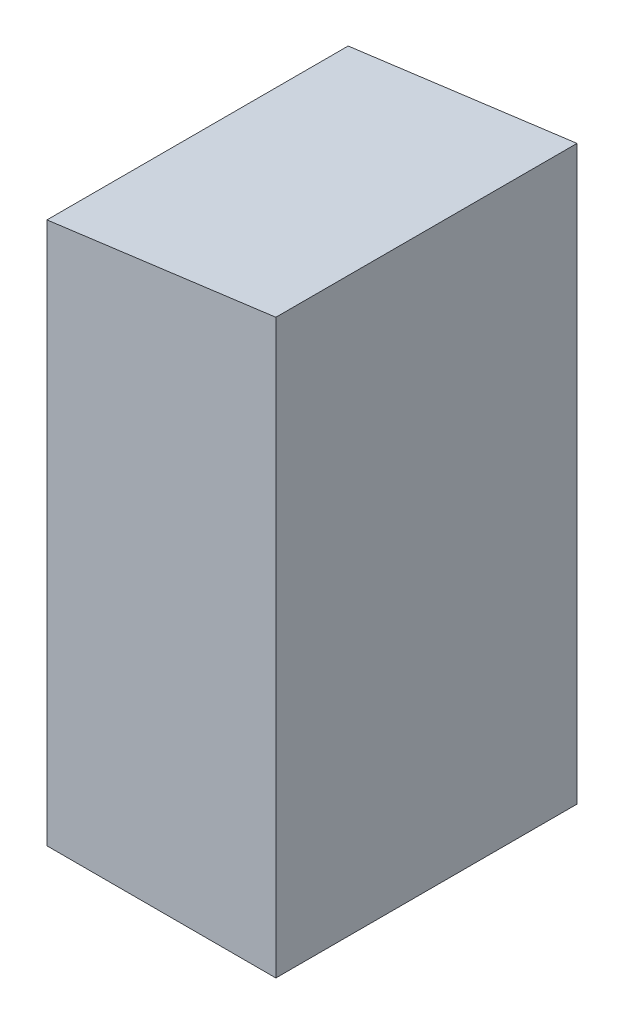
from build123d import *

# Parameters (mm, degrees)
BOSS_EXTRUDE1_DEPTH = 25


with BuildPart() as part:
    # Sketch1 → Boss-Extrude1 (new body)
    with BuildSketch(Plane.XY):
        Polygon((0, 45), (19, 47.5), (19, 0), (0, 0), align=None)
    extrude(amount=BOSS_EXTRUDE1_DEPTH)


solid = part.part
